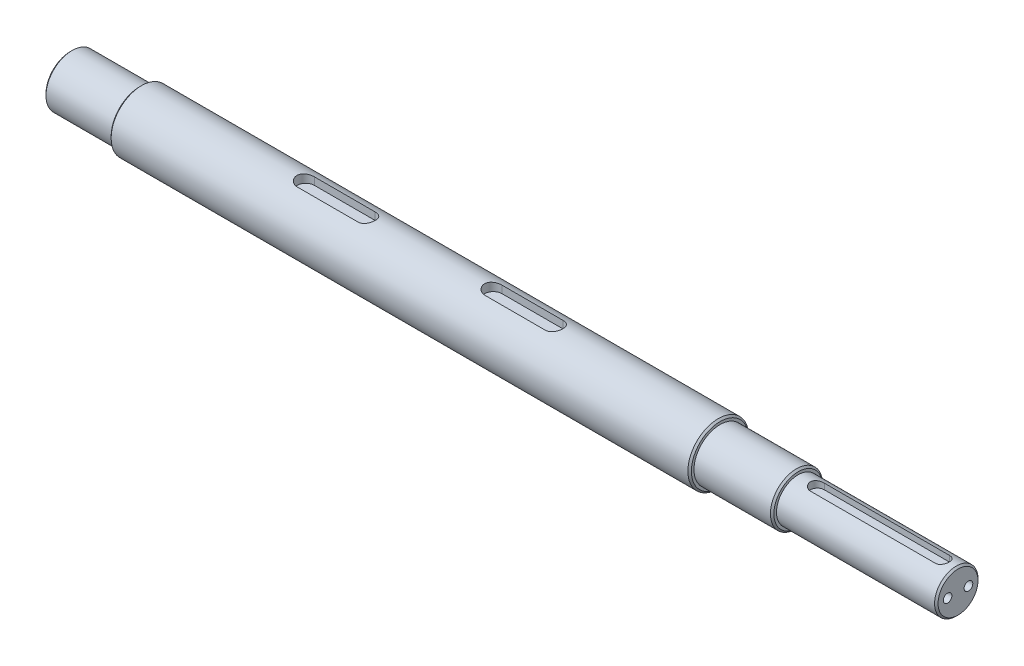
SolidWorks part; units mm, degrees
material "热轧圆钢 45"
ref_plane "前视基准面" through (0, 0, 0) normal (0, 0, 1) x (1, 0, 0)
ref_plane "上视基准面" through (0, 0, 0) normal (0, 1, 0) x (1, 0, 0)
ref_plane "右视基准面" through (0, 0, 0) normal (1, 0, 0) x (0, 0, -1)
sketch "草图1" plane through (0, 0, 0) normal (0, 0, 1) x (1, 0, 0)
  line L0 (0, 0) -> (0, 64.6076) construction
  line L1 (0, 0) -> (465.6931, 0) construction
  line L2 (167, 17.5) -> (0, 17.5)
  line L3 (167, 17.5) -> (167, 15)
  line L4 (167, 15) -> (212, 15)
  line L5 (212, 15) -> (212, 12.5)
  line L6 (212, 12.5) -> (304, 12.5)
  line L7 (304, 12.5) -> (304, 0)
  line L8 (0, 0) -> (-387.5035, 0) construction
  line L9 (-167, 17.5) -> (-167, 15)
  line L10 (-167, 15) -> (-207, 15)
  line L11 (-207, 15) -> (-207, 0)
  line L12 (304, 0) -> (-207, 0)
  line L21 (0, 17.5) -> (-167, 17.5)
  point P15 (0, 17.5)
  dimension "D1" = 334
  dimension "D2" = 40
  dimension "D3" = 45
  dimension "D4" = 92
  dimension "D5" = 17.5
  dimension "D6" = 15
  dimension "D7" = 15
  dimension "D8" = 12.5
  dimension "D12" = 167
revolve "旋转1" add sketch "草图1" angle 360 about L8
ref_plane "基准面1" through (0, 17.5, 0) normal (0, 1, 0) x (1, 0, 0)
sketch "草图2" plane through (0, 17.5, 0) normal (0, 1, 0) x (1, 0, 0)
  line L0 (0, 0) -> (0, 80.884) construction
  line L1 (0, 0) -> (54, 0) construction
  line L2 (36.5, 0) -> (71.5, 0) construction
  line L3 (36.5, 5) -> (71.5, 5)
  line L4 (36.5, -5) -> (71.5, -5)
  line L5 (-36.5, 0) -> (-71.5, 0) construction
  line L6 (-36.5, 5) -> (-71.5, 5)
  line L7 (-36.5, -5) -> (-71.5, -5)
  arc A0 (36.5, 5) -> (36.5, -5) centre (36.5, 0) ccw
  arc A1 (71.5, -5) -> (71.5, 5) centre (71.5, 0) ccw
  arc A2 (-36.5, 5) -> (-36.5, -5) centre (-36.5, 0) cw
  arc A3 (-71.5, -5) -> (-71.5, 5) centre (-71.5, 0) cw
  point P6 (54, 0)
  point P13 (-54, 0)
  dimension "D1" = 5
  dimension "D3" = 35
  dimension "D2" = 54
extrude "切除-拉伸1" cut sketch "草图2" against normal blind 5
ref_plane "基准面2" through (0, 12.5, 0) normal (0, 1, 0) x (1, 0, 0)
sketch "草图3" plane through (0, 12.5, 0) normal (0, 1, 0) x (1, 0, 0)
  line L0 (0, 0) -> (259, 0) construction
  line L1 (223, 0) -> (295, 0) construction
  line L2 (223, 4) -> (295, 4)
  line L3 (223, -4) -> (295, -4)
  line L4 (304, -12.5) -> (304, 12.5) construction
  arc A0 (223, 4) -> (223, -4) centre (223, 0) ccw
  arc A1 (295, -4) -> (295, 4) centre (295, 0) ccw
  point P5 (259, 0)
  dimension "D1" = 4
  dimension "D2" = 9
  dimension "D3" = 72
extrude "切除-拉伸2" cut sketch "草图3" against normal blind 4
chamfer "倒角1" distance 1 angle 45 5 edges at (304, 0, -12.5) (212, 0, -15) (167, 0, -17.5) (-207, 0, -15) (-167, 0, -17.5)
hole_wizard "M6 螺纹孔1" positions "草图5" profile "草图4" tap size "M6" standard "Gb"
sketch "草图5" plane through (304, 0, 0) normal (1, 0, 0) x (0, 0, -1)
  point P0 (6, 0)
  point P2 (-6, 0)
  dimension "D1" = 6
  dimension "D2" = 6
sketch "草图4" plane through (304, 0, -6) normal (0, 1, 0) x (0, 0, -1)
  line L0 (0, 0) -> (0, 21.5022)
  line L1 (0, 21.5022) -> (2.5, 20)
  line L2 (2.5, 20) -> (2.5, 0)
  line L5 (2.5, 0) -> (0, 0)
  line L10 (0, 21.5022) -> (-2.5, 20) construction
  line L11 (0, -6.35) -> (0, 107.95) construction
  dimension "螺纹孔钻头直径" = 5
  dimension "螺纹孔钻头深度" = 20
  dimension "导头角度" = 118
